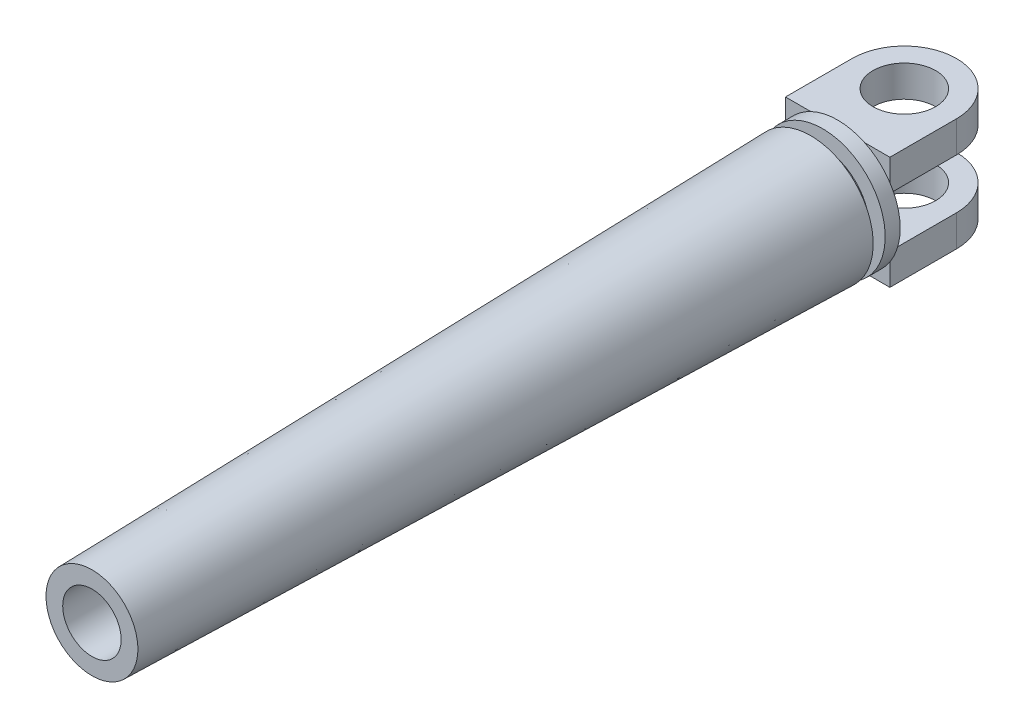
from build123d import *

# Parameters (mm, degrees)
SKETCH2_R           = 15
BOSS_EXTRUDE1_DEPTH = 15


with BuildPart() as part:
    # Sketch2 → Boss-Extrude1 (new body)
    with BuildSketch(Plane(origin=(0, 0, 0), x_dir=(1, 0, 0), z_dir=(0, 1, 0))):
        with BuildLine():
            Line((25, 0), (25, -31.912942224))
            Line((25, -31.912942224), (-25, -31.912942224))
            Line((-25, -31.912942224), (-25, 0))
            ThreePointArc((-25, 0), (0, 25), (25, 0))
        make_face()
        with Locations(Location((0, 0, 0), (0, 0, 270))):
            Circle(SKETCH2_R, mode=Mode.SUBTRACT)
    boss_extrude1 = extrude(amount=BOSS_EXTRUDE1_DEPTH)

    # Sketch4 → Revolve1 (revolve)
    with BuildSketch(Plane(origin=(0, -12, 0), x_dir=(-1, 0, 0), z_dir=(0, -1, 0))):
        Polygon((0, -31.912942224), (29.933248422, -31.912942224), (29.933248422, -39.086469166), (22.382657632, -39.086469166), (22.382657632, -44.842453341), (29.933248422, -44.842453341), (22, -389.086469166), (14, -389.086469166), (14, -39.086469166), (0, -39.086469166), align=None)
    revolve(axis=Axis((0, -12, 31.912942224), (0, 0, 1)))

    # Mirror5: Boss-Extrude1 across plane
    add(boss_extrude1.mirror(Plane(origin=(0, -12, 0), x_dir=(0, 0, 1), z_dir=(0, -1, 0))))


solid = part.part
